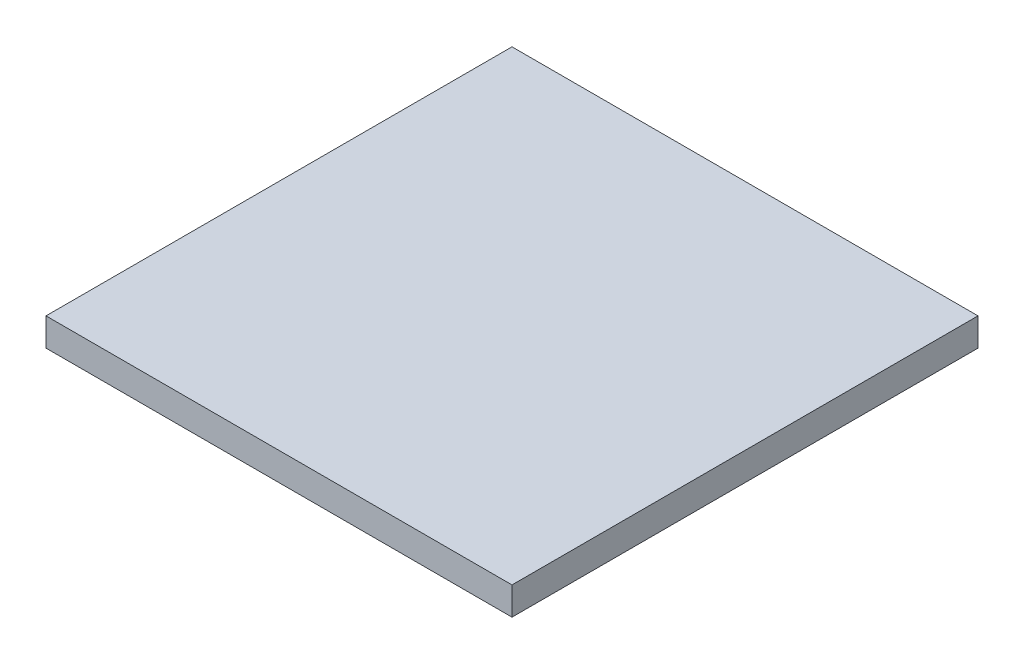
from build123d import *

# Parameters (mm, degrees)
SKETCH1_W           = 50
SKETCH1_H           = 50
BOSS_EXTRUDE1_DEPTH = 3


with BuildPart() as part:
    # Sketch1 → Boss-Extrude1 (new body)
    with BuildSketch(Plane(origin=(0, 0, 0), x_dir=(1, 0, 0), z_dir=(0, 1, 0))):
        Rectangle(SKETCH1_W, SKETCH1_H)
    extrude(amount=BOSS_EXTRUDE1_DEPTH)


solid = part.part
